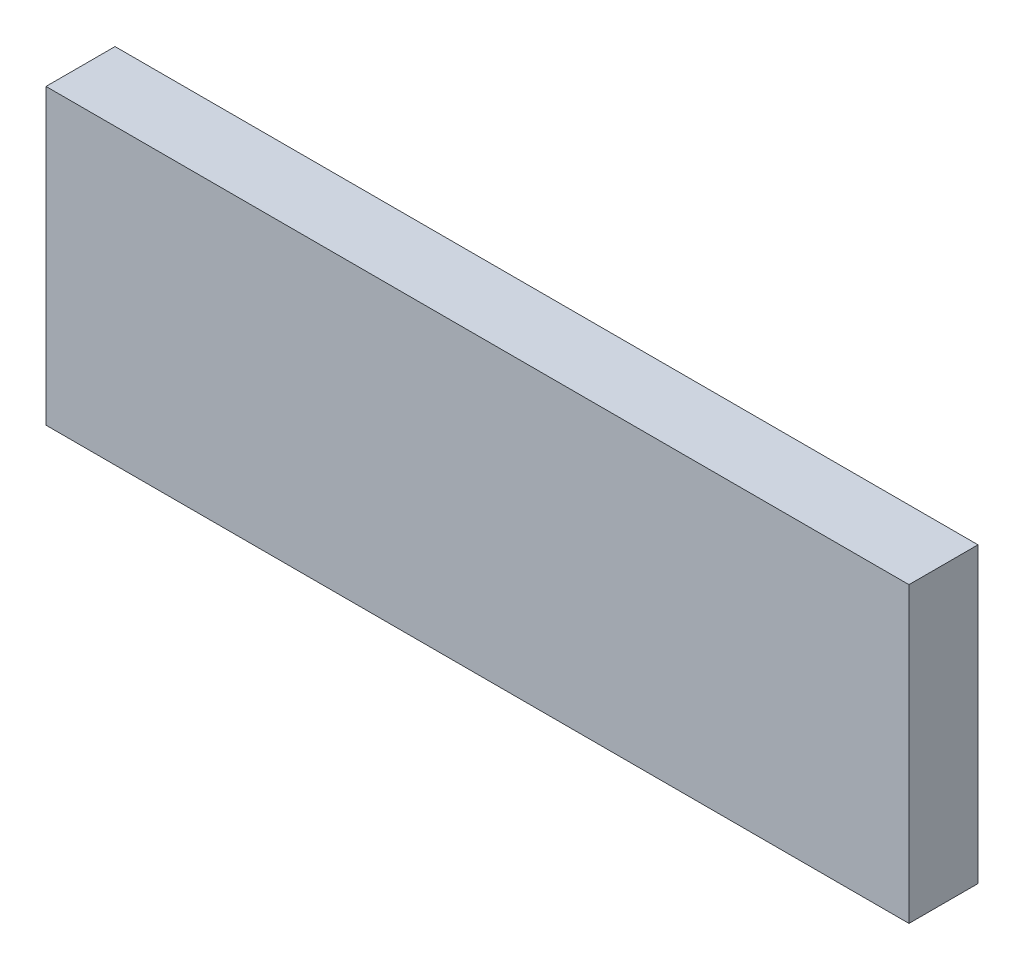
from build123d import *

# Parameters (mm, degrees)
SKETCH1_W           = 200
SKETCH1_H           = 68
BOSS_EXTRUDE1_DEPTH = 16


with BuildPart() as part:
    # Sketch1 → Boss-Extrude1 (new body)
    with BuildSketch(Plane.XY):
        with Locations((100, 34)):
            Rectangle(SKETCH1_W, SKETCH1_H)
    extrude(amount=BOSS_EXTRUDE1_DEPTH)


solid = part.part
